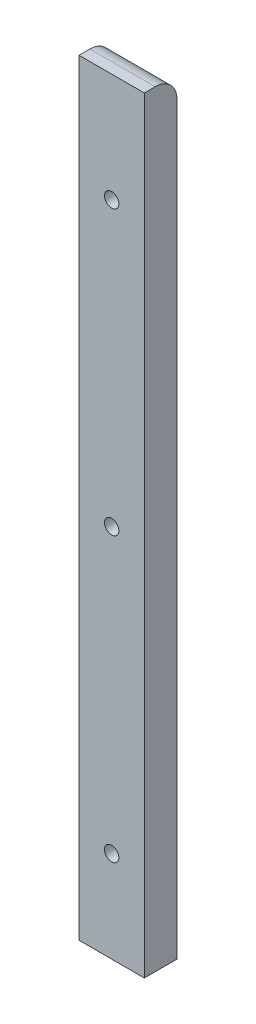
from build123d import *

# Parameters (mm, degrees)
SKETCH_1_W                = 30
SKETCH_1_H                = 352
EXTRUDE_1_DEPTH           = 15
HOLE_WIZARD_1_D           = 6.6
HOLE_WIZARD_1_CBORE_D     = 11
HOLE_WIZARD_1_CBORE_DEPTH = 6.8
FILLET_1_R                = 10


with BuildPart() as part:
    # 草图1 → 凸台-拉伸1 (new body)
    with BuildSketch(Plane.XY):
        Rectangle(SKETCH_1_W, SKETCH_1_H)
    extrude(amount=EXTRUDE_1_DEPTH)

    # 打孔尺寸(%根据)内六角圆柱头螺钉的类型1 (through all)
    with Locations(Plane(origin=(0, 0, 0), x_dir=(-1, 0, 0), z_dir=(0, 0, -1))):
        with Locations((0, 126), (0, -4), (0, -134)):
            CounterBoreHole(HOLE_WIZARD_1_D / 2, HOLE_WIZARD_1_CBORE_D / 2, HOLE_WIZARD_1_CBORE_DEPTH)

    # 圆角1
    fillet_1_edges = [part.edges().sort_by_distance(p)[0] for p in [
        (0, 176, 0),
    ]]
    fillet(fillet_1_edges, radius=FILLET_1_R)


solid = part.part
